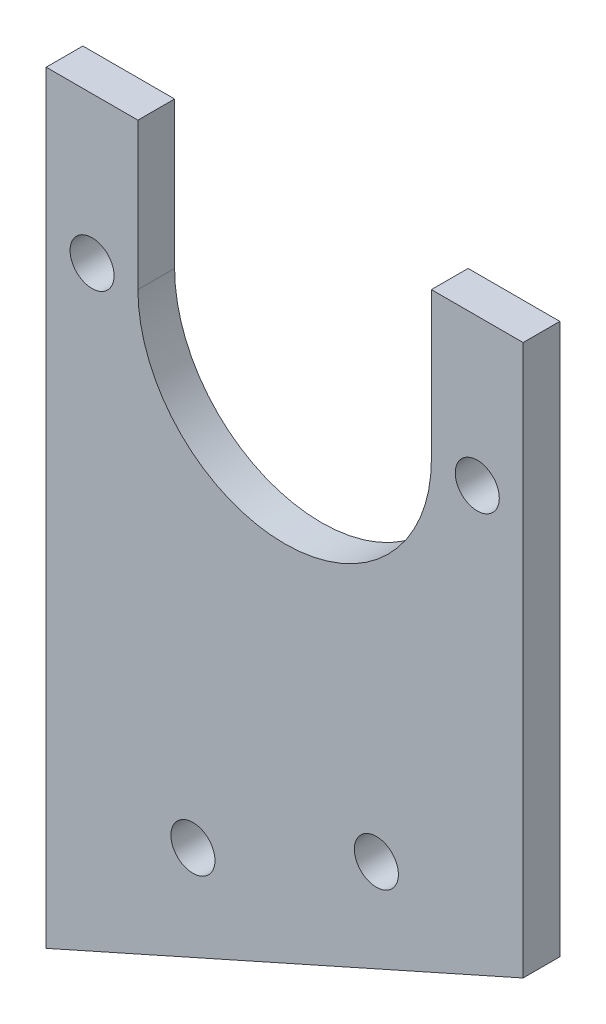
from build123d import *

# Parameters (mm, degrees)
SKETCH_1_R      = 6
EXTRUDE_1_DEPTH = 10


with BuildPart() as part:
    # 草图1 → 凸台-拉伸1 (new body)
    with BuildSketch(Plane.XY):
        with BuildLine():
            Line((130, 208), (130, 58))
            Line((130, 58), (0, 0))
            Line((0, 0), (0, 208))
            Line((0, 208), (25, 208))
            Line((25, 208), (25, 168))
            ThreePointArc((25, 168), (65, 128), (105, 168))
            Line((105, 168), (105, 208))
            Line((105, 208), (130, 208))
        make_face()
        with Locations((117.5, 168)):
            Circle(SKETCH_1_R, mode=Mode.SUBTRACT)
        with Locations((12.5, 168)):
            Circle(SKETCH_1_R, mode=Mode.SUBTRACT)
        with Locations((40, 43.72)):
            Circle(SKETCH_1_R, mode=Mode.SUBTRACT)
        with Locations((90, 65.43)):
            Circle(SKETCH_1_R, mode=Mode.SUBTRACT)
    extrude(amount=EXTRUDE_1_DEPTH)


solid = part.part
